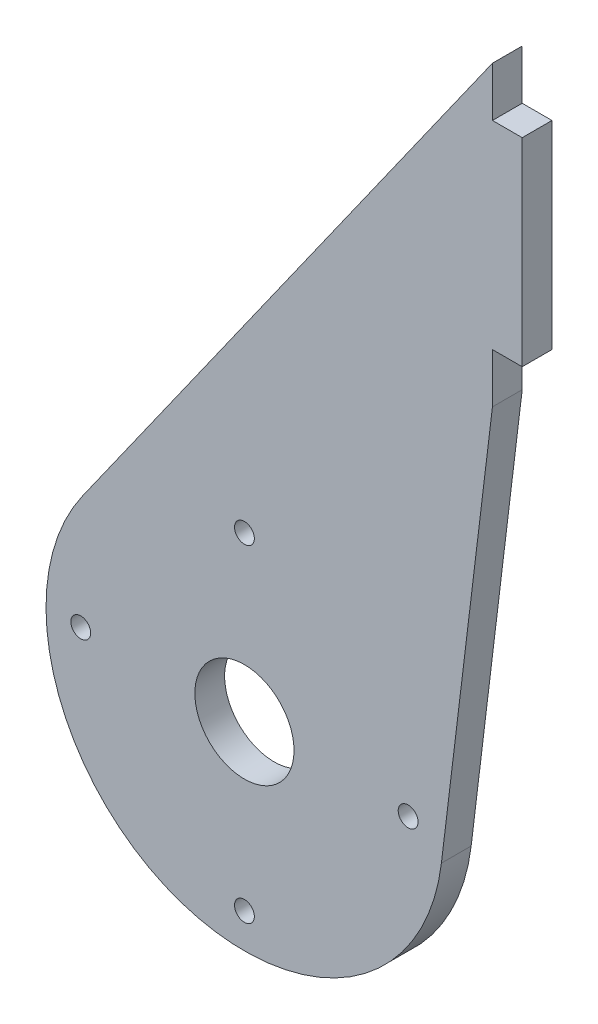
from build123d import *

# Parameters (mm, degrees)
BOSS_EXTRUDE1_DEPTH = 3
SKETCH2_R           = 5
CUT_EXTRUDE1_DEPTH  = 10
SKETCH4_W           = 3
SKETCH4_H           = 20
BOSS_EXTRUDE3_DEPTH = 3
SKETCH5_R           = 1
CUT_EXTRUDE2_DEPTH  = 10


with BuildPart() as part:
    # Sketch1 → Boss-Extrude1 (new body)
    with BuildSketch(Plane.XY):
        with BuildLine():
            Line((-16.33027103, 11.546525368), (25, 70))
            Line((25, 70), (25, 40))
            Line((25, 40), (19.854388756, -2.408992972))
            ThreePointArc((19.854388756, -2.408992972), (-7.196803073, -18.660279353), (-16.33027103, 11.546525368))
        make_face()
    extrude(amount=-BOSS_EXTRUDE1_DEPTH)

    # Sketch2 → Cut-Extrude1 (cut)
    with BuildSketch(Plane.XY):
        Circle(SKETCH2_R)
    extrude(amount=-CUT_EXTRUDE1_DEPTH, mode=Mode.SUBTRACT)

    # Sketch4 → Boss-Extrude3 (add)
    with BuildSketch(Plane(origin=(25, 0, 0), x_dir=(0, 0, -1), z_dir=(1, 0, 0))):
        with Locations((1.5, 55)):
            Rectangle(SKETCH4_W, SKETCH4_H)
    extrude(amount=BOSS_EXTRUDE3_DEPTH)

    # Sketch5 → Cut-Extrude2 (cut)
    with BuildSketch(Plane.XY):
        with Locations((0, 16.5)):
            Circle(SKETCH5_R)
        with Locations((0, -16.5)):
            Circle(SKETCH5_R)
        with Locations((16.5, 0)):
            Circle(SKETCH5_R)
        with Locations((-16.5, 0)):
            Circle(SKETCH5_R)
    extrude(amount=-CUT_EXTRUDE2_DEPTH, mode=Mode.SUBTRACT)


solid = part.part
